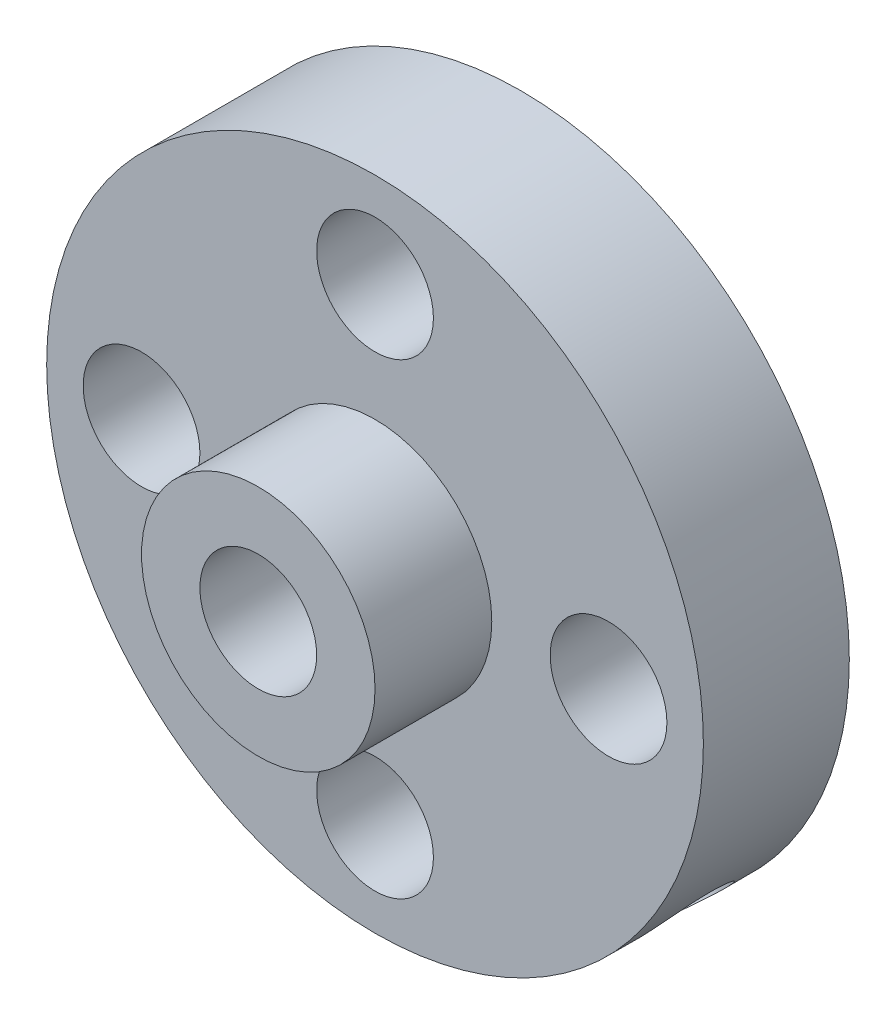
from build123d import *

# Parameters (mm, degrees)
SKETCH1_R           = 11.25
SKETCH1_R_2         = 2
BOSS_EXTRUDE1_DEPTH = 5
SKETCH2_R           = 4
SKETCH2_R_2         = 2
BOSS_EXTRUDE2_DEPTH = 4
CUT_EXTRUDE1_DEPTH  = 10


with BuildPart() as part:
    # Sketch1 → Boss-Extrude1 (new body)
    with BuildSketch(Plane.XY):
        Circle(SKETCH1_R)
        with Locations((0, 8)):
            Circle(SKETCH1_R_2, mode=Mode.SUBTRACT)
        with Locations((8, 0)):
            Circle(SKETCH1_R_2, mode=Mode.SUBTRACT)
        with Locations((0, -8)):
            Circle(SKETCH1_R_2, mode=Mode.SUBTRACT)
        with Locations((-8, 0)):
            Circle(SKETCH1_R_2, mode=Mode.SUBTRACT)
        Circle(SKETCH1_R_2, mode=Mode.SUBTRACT)
    extrude(amount=BOSS_EXTRUDE1_DEPTH)

    # Sketch2 → Boss-Extrude2 (add)
    with BuildSketch(Plane.XY.offset(5)):
        Circle(SKETCH2_R)
        Circle(SKETCH2_R_2, mode=Mode.SUBTRACT)
    extrude(amount=BOSS_EXTRUDE2_DEPTH)

    # Sketch4 → Cut-Extrude1 (cut)
    with BuildSketch(Plane(origin=(7.954951288, -7.954951288, 0), x_dir=(-0.7071067811865475, -0.7071067811865477, 0), z_dir=(0.7071067811865477, -0.7071067811865475, 0))):
        with BuildLine():
            ThreePointArc((1.5, -2.45834938), (1.060660172, -1.397689208), (0, -0.95834938))
            Line((0, -0.95834938), (0, -3.95834938))
            ThreePointArc((0, -3.95834938), (1.060660172, -3.519009552), (1.5, -2.45834938))
        make_face()
        with BuildLine():
            Line((0, -3.95834938), (0, -0.95834938))
            ThreePointArc((0, -0.95834938), (-1.5, -2.45834938), (0, -3.95834938))
        make_face()
    extrude(amount=-CUT_EXTRUDE1_DEPTH, mode=Mode.SUBTRACT)


solid = part.part
